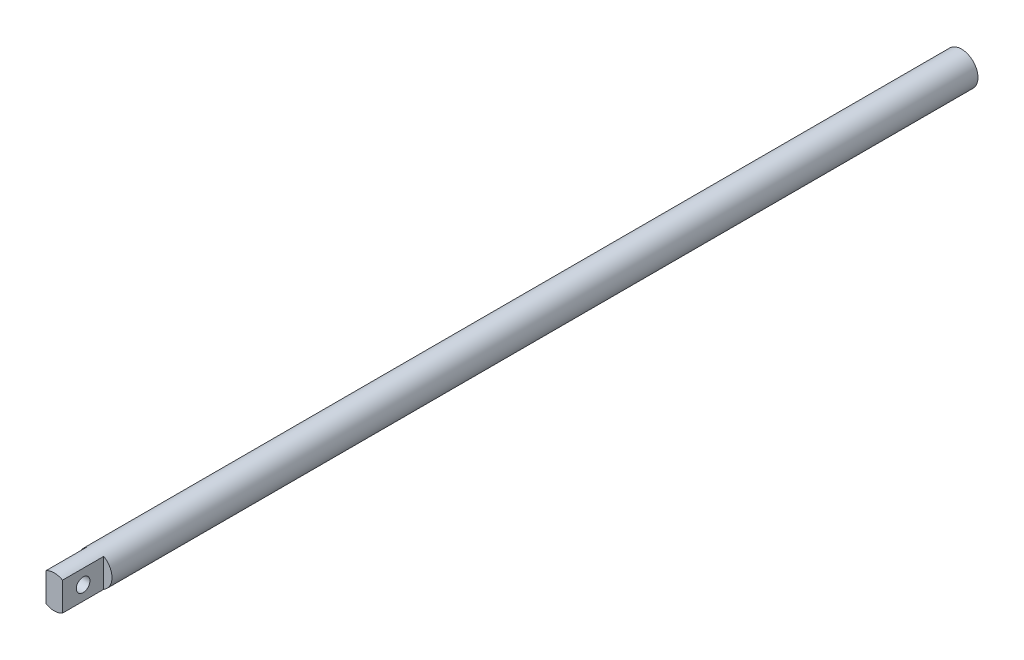
SolidWorks part; units mm, degrees
material "K"
ref_plane "Front" through (0, 0, 0) normal (0, 0, 1) x (1, 0, 0)
ref_plane "Top" through (0, 0, 0) normal (0, 1, 0) x (1, 0, 0)
ref_plane "Right" through (0, 0, 0) normal (1, 0, 0) x (0, 0, -1)
sketch "Sketch1" plane through (0, 0, 0) normal (0, 0, 1) x (1, 0, 0)
  circle A0 centre (0, 0) radius 20
  dimension "D1" = 40
extrude "Boss-Extrude1" add sketch "Sketch1" along normal blind 1100
cosmetic thread "Cosmetic Thread1" parameters "D1"=1020, "D2"=36.835
sketch "Sketch2" plane through (0, 0, 0) normal (0, 1, 0) x (1, 0, 0)
  line L0 (0, -1100) -> (0, -1078.1049) construction
  line L1 (-20, -1100) -> (20, -1100) construction
  line L2 (-10, -1100) -> (-10, -1050)
  line L3 (20, -1100) -> (10, -1100)
  line L4 (20, -1100) -> (20, -1050)
  line L5 (20, -1050) -> (10, -1050)
  line L6 (10, -1100) -> (10, -1050)
  line L7 (-20, -1050) -> (-10, -1050)
  line L8 (-20, -1100) -> (-20, -1050)
  line L9 (-20, -1100) -> (-10, -1100)
  dimension "D1" = 20
  dimension "D2" = 50
extrude "Cut-Extrude1" cut sketch "Sketch2" against normal through all both and the other way through all
sketch "Sketch3" plane through (-10, 0, 0) normal (-1, 0, 0) x (0, 0, 1)
  line L0 (1100, 17.3205) -> (1100, -17.3205) construction
  circle A0 centre (1075, 0) radius 8.25
  dimension "D1" = 16.5
  dimension "D2" = 25
extrude "Cut-Extrude2" cut sketch "Sketch3" against normal through all both and the other way through all
equation "\"零件重量\"= IIF ( \"SW-质量\" > 100 , int ( \"SW-质量\" ) , \"SW-质量\" )"
